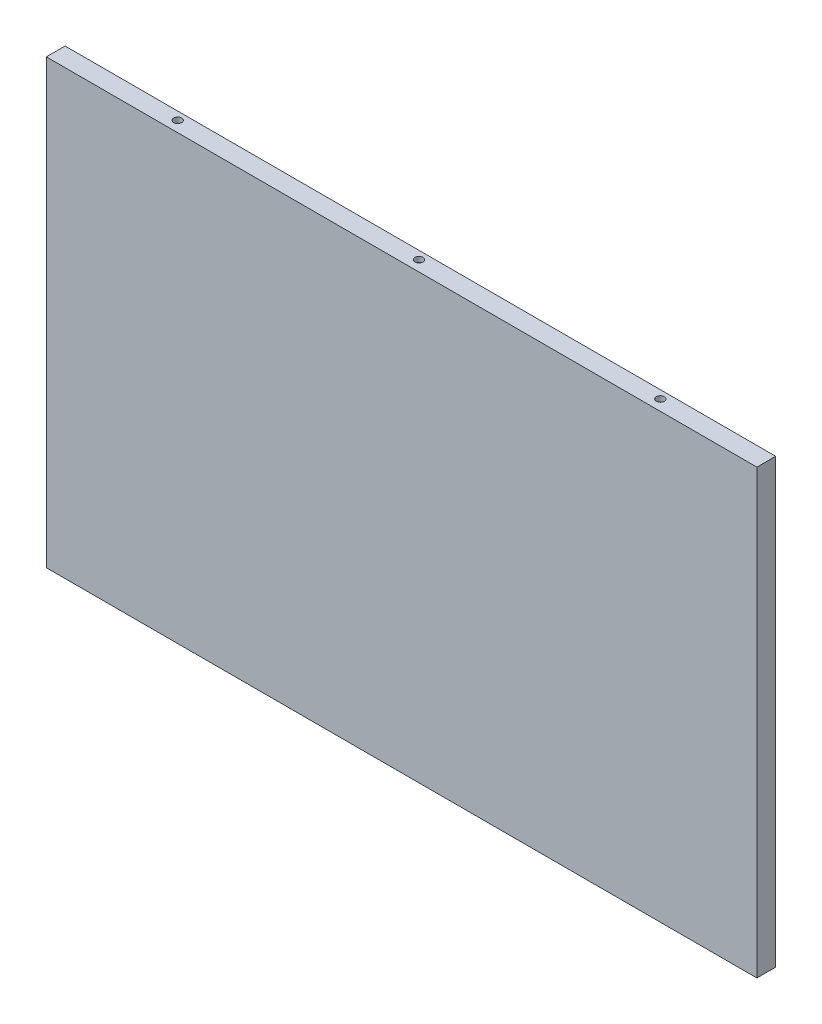
SolidWorks part; units mm, degrees
ref_plane "Front Plane" through (0, 0, 0) normal (0, 0, 1) x (1, 0, 0)
ref_plane "Top Plane" through (0, 0, 0) normal (0, 1, 0) x (1, 0, 0)
ref_plane "Right Plane" through (0, 0, 0) normal (1, 0, 0) x (0, 0, -1)
sketch "Sketch1" plane through (0, 0, 0) normal (0, 0, 1) x (1, 0, 0)
  line L1 (0, 0) -> (265, 0)
  line L2 (0, 0) -> (0, 165)
  line L3 (0, 165) -> (265, 165)
  line L4 (265, 0) -> (265, 165)
  dimension "D1" = 265
  dimension "D2" = 165
extrude "Boss-Extrude1" add sketch "Sketch1" along normal blind 2
sketch "Sketch2" plane through (0, 0, 0) normal (0, 0, -1) x (-1, 0, 0)
  line L0 (-2, 163) -> (-263, 163)
  line L1 (-263, 163) -> (-263, 2)
  line L2 (-263, 2) -> (-2, 2)
  line L3 (-2, 2) -> (-2, 163)
  line L4 (0, 0) -> (0, 165)
  line L5 (0, 165) -> (-265, 165)
  line L6 (-265, 165) -> (-265, 0)
  line L7 (-265, 0) -> (0, 0)
  line L8 (0, 0) -> (0, 165)
  line L9 (0, 165) -> (-265, 165)
  line L10 (-265, 165) -> (-265, 0)
  line L11 (-265, 0) -> (0, 0)
  dimension "D1" = 0
  dimension "D2" = 2
extrude "Boss-Extrude2" add sketch "Sketch2" along normal blind 5
sketch "Sketch3" plane through (0, 165, 0) normal (0, 1, 0) x (1, 0, 0)
  line L0 (265, -2) -> (265, 5) construction
  line L1 (0, 5) -> (265, 5) construction
  circle A0 centre (225, 2) radius 1.5
  dimension "D1" = 3
  dimension "D2" = 40
  dimension "D3" = 3
extrude "Cut-Extrude1" cut sketch "Sketch3" against normal through all
pattern_linear "LPattern1" count 3 spacing 90 along (-1, 0, 0) of "Cut-Extrude1"
